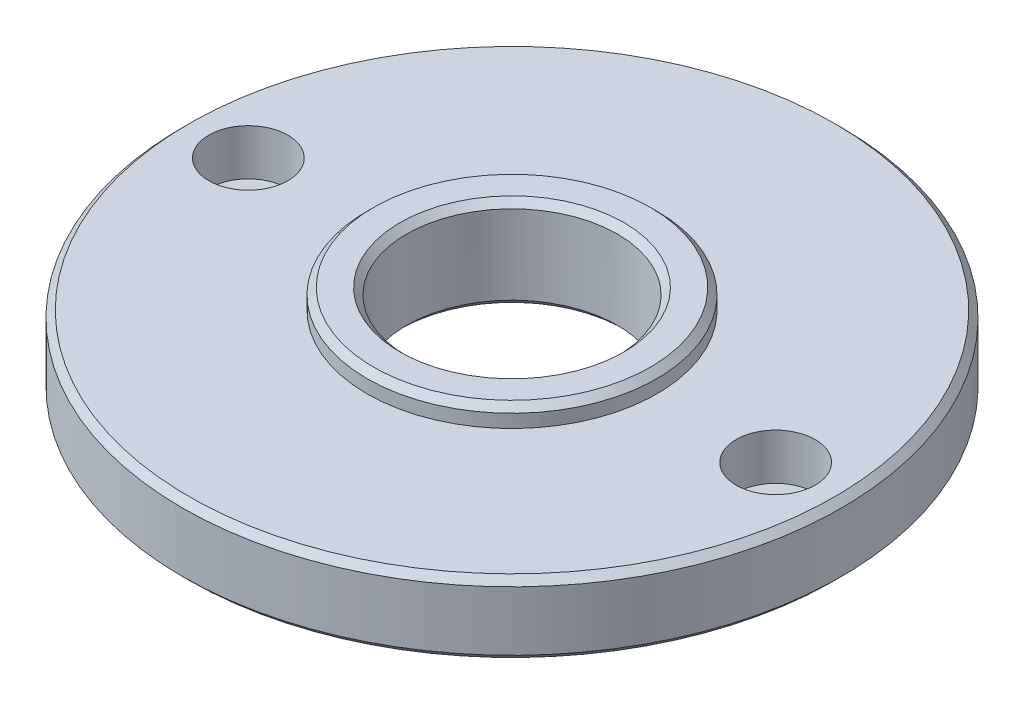
from build123d import *

# Parameters (mm, degrees)
CBORE_FOR_M3_HEX_HEAD_BOLT1_D           = 3.5
CBORE_FOR_M3_HEX_HEAD_BOLT1_CBORE_D     = 6
CBORE_FOR_M3_HEX_HEAD_BOLT1_CBORE_DEPTH = 3.5
CHAMFER1_SIZE                           = 0.5


with BuildPart() as part:
    # Sketch1 → Revolve1 (revolve)
    with BuildSketch(Plane.XY, mode=Mode.PRIVATE) as revolve1_sk:
        Polygon((8, 0), (25, 0), (25, 5.5), (11, 5.5), (11, 7), (8, 7), align=None)
    revolve(revolve1_sk.sketch.rotate(Axis((0, 21.458333333, 0), (0, -1, 0)), 90), axis=Axis((0, 21.458333333, 0), (0, -1, 0)))

    # CBORE for M3 Hex Head Bolt1 (through all)
    with Locations(Plane(origin=(-20, 5.5, 0), x_dir=(0, 0, 1), z_dir=(0, 1, 0))):
        with Locations((0, 0), (0, 40)):
            CounterBoreHole(CBORE_FOR_M3_HEX_HEAD_BOLT1_D / 2, CBORE_FOR_M3_HEX_HEAD_BOLT1_CBORE_D / 2, CBORE_FOR_M3_HEX_HEAD_BOLT1_CBORE_DEPTH)

    # Chamfer1
    chamfer1_edges = [part.edges().sort_by_distance(p)[0] for p in [
        (0, 0, -25),
        (0, 0, -8),
        (0, 7, -8),
        (0, 7, -11),
        (0, 5.5, -25),
    ]]
    chamfer(chamfer1_edges, length=CHAMFER1_SIZE)


solid = part.part
